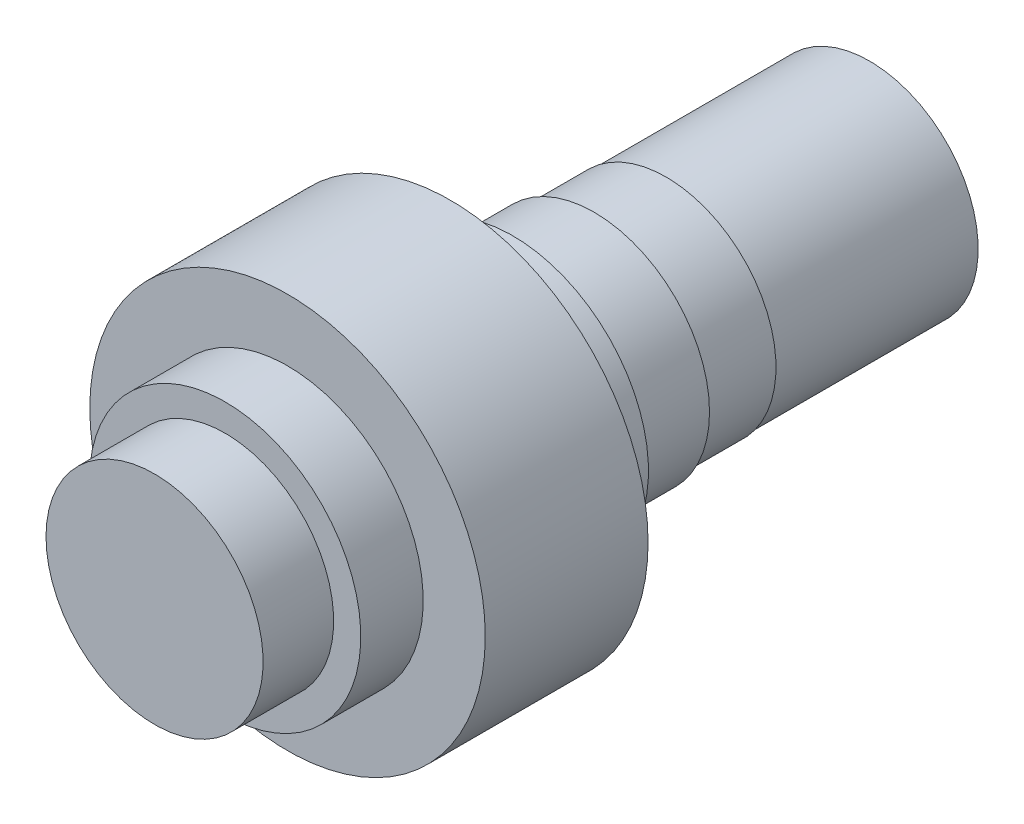
SolidWorks part; units mm, degrees
ref_plane "Front Plane" through (0, 0, 0) normal (0, 0, 1) x (1, 0, 0)
ref_plane "Top Plane" through (0, 0, 0) normal (0, 1, 0) x (1, 0, 0)
ref_plane "Right Plane" through (0, 0, 0) normal (1, 0, 0) x (0, 0, -1)
sketch "Sketch1" plane through (0, 0, 0) normal (0, 0, 1) x (1, 0, 0)
  circle A0 centre (0, 0) radius 40
  dimension "D1" = 80
extrude "Boss-Extrude1" add sketch "Sketch1" along normal blind 26
sketch "Sketch2" plane through (0, 0, 0) normal (0, 0, -1) x (-1, 0, 0)
  circle A0 centre (0, 0) radius 50
  dimension "D1" = 100
extrude "Boss-Extrude2" add sketch "Sketch2" along normal blind 23
sketch "Sketch3" plane through (0, 0, -23) normal (0, 0, -1) x (-1, 0, 0)
  circle A0 centre (0, 0) radius 72.8615
  dimension "D1" = 145.723
extrude "Boss-Extrude3" add sketch "Sketch3" along normal blind 60
sketch "Sketch4" plane through (0, 0, -83) normal (0, 0, -1) x (-1, 0, 0)
  circle A0 centre (0, 0) radius 50
  dimension "D1" = 100
extrude "Boss-Extrude4" add sketch "Sketch4" along normal blind 23
sketch "Sketch6" plane through (0, 0, -106) normal (0, 0, -1) x (-1, 0, 0)
  circle A0 centre (0, 0) radius 42.5
  dimension "D1" = 85
extrude "Boss-Extrude5" add sketch "Sketch6" along normal blind 30
sketch "Sketch7" plane through (0, 0, -136) normal (0, 0, -1) x (-1, 0, 0)
  circle A0 centre (0, 0) radius 40.5
  dimension "D1" = 81
extrude "Boss-Extrude6" add sketch "Sketch7" along normal blind 26.5
sketch "Sketch8" plane through (0, 0, -162.5) normal (0, 0, -1) x (-1, 0, 0)
  circle A0 centre (0, 0) radius 40
  dimension "D1" = 80
extrude "Boss-Extrude7" add sketch "Sketch8" along normal blind 75
